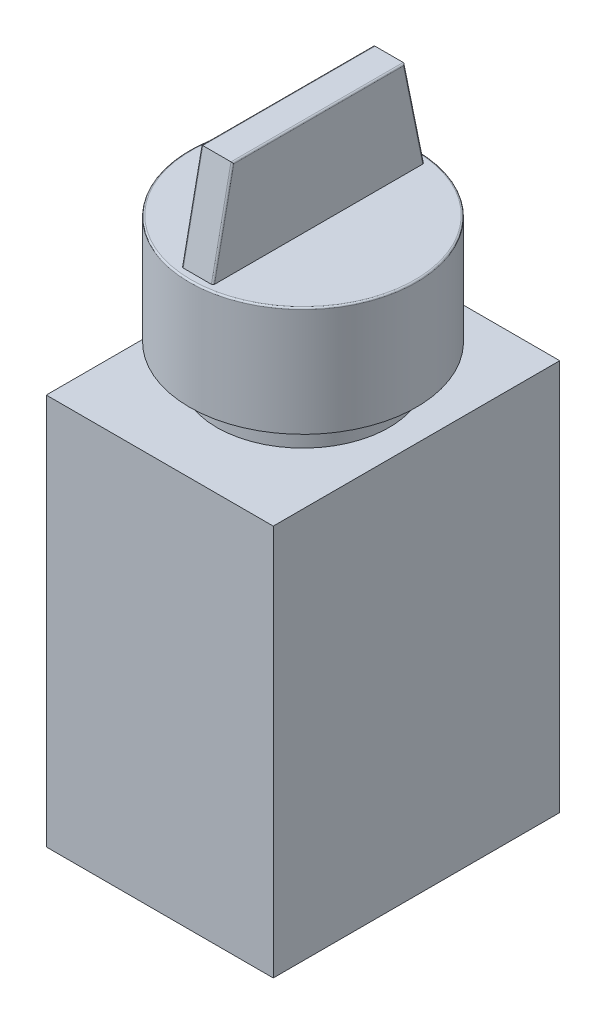
from build123d import *

# Parameters (mm, degrees)
SKETCH2_R           = 14.5
BOSS_EXTRUDE1_DEPTH = 14
SKETCH3_W           = 4
SKETCH3_H           = 27
BOSS_EXTRUDE2_DEPTH = 12.3
CUT_EXTRUDE1_DEPTH  = 12.3
SKETCH5_R           = 11
BOSS_EXTRUDE3_DEPTH = 4
SKETCH6_W           = 29
SKETCH6_H           = 36.6
BOSS_EXTRUDE4_DEPTH = 50
FILLET1_R           = 0.2


with BuildPart() as part:
    # Sketch2 → Boss-Extrude1 (new body)
    with BuildSketch(Plane(origin=(0, 0, 0), x_dir=(1, 0, 0), z_dir=(0, 1, 0))):
        with Locations(Location((0, 0, 0), (0, 0, 270))):
            Circle(SKETCH2_R)
    extrude(amount=BOSS_EXTRUDE1_DEPTH)

    # Sketch3 → Boss-Extrude2 (add)
    with BuildSketch(Plane(origin=(0, 14, 0), x_dir=(1, 0, 0), z_dir=(0, 1, 0))):
        Rectangle(SKETCH3_W, SKETCH3_H)
    extrude(amount=BOSS_EXTRUDE2_DEPTH)

    # Sketch4 → Cut-Extrude1 (cut)
    with BuildSketch(Plane(origin=(2, 0, 0), x_dir=(0, 0, -1), z_dir=(1, 0, 0))):
        Polygon((-13.5, 26.3), (-13.5, 14), (-11, 26.3), align=None)
        Polygon((11, 26.3), (13.5, 26.3), (13.5, 14), align=None)
    extrude(amount=-CUT_EXTRUDE1_DEPTH, mode=Mode.SUBTRACT)

    # Sketch5 → Boss-Extrude3 (add)
    with BuildSketch(Plane.XZ):
        with Locations(Location((0, 0, 0), (0, 0, 90))):
            Circle(SKETCH5_R)
    extrude(amount=BOSS_EXTRUDE3_DEPTH)

    # Sketch6 → Boss-Extrude4 (add)
    with BuildSketch(Plane.XZ.offset(4)):
        Rectangle(SKETCH6_W, SKETCH6_H)
    extrude(amount=BOSS_EXTRUDE4_DEPTH)

    # Fillet1
    fillet1_edges = [part.edges().sort_by_distance(p)[0] for p in [
        (2, 26.3, 0),
        (-2, 20.15, 12.25),
        (2, 20.15, 12.25),
        (-2, 26.3, 0),
        (-2, 20.15, -12.25),
        (2, 20.15, -12.25),
        (0, 14, -14.5),
    ]]
    fillet(fillet1_edges, radius=FILLET1_R)


solid = part.part
